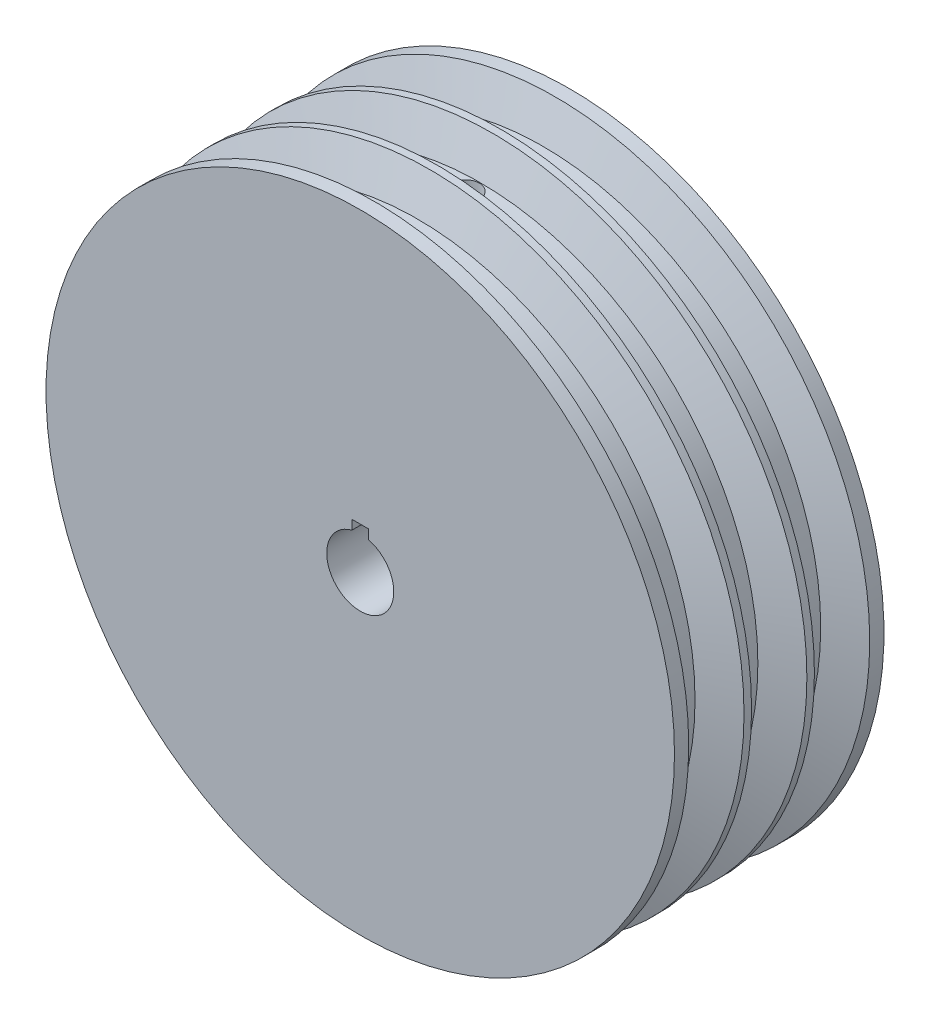
from build123d import *

# Parameters (mm, degrees)
SKETCH1_R           = 75
BOSS_EXTRUDE1_DEPTH = 40
SKETCH2_R           = 8
CUT_EXTRUDE1_DEPTH  = 150
SKETCH10_R          = 100
CUT_EXTRUDE5_DEPTH  = 20
SKETCH11_R          = 30
SKETCH11_R_2        = 8
BOSS_EXTRUDE2_DEPTH = 20
SKETCH12_R          = 130
CUT_EXTRUDE6_DEPTH  = 30
SKETCH13_W          = 4
SKETCH13_H          = 4
CUT_EXTRUDE7_DEPTH  = 500
SKETCH15_W          = 3.4
SKETCH15_H          = 65


with BuildPart() as part:
    # Sketch1 → Boss-Extrude1 (new, symmetric)
    with BuildSketch(Plane.XY):
        Circle(SKETCH1_R)
    extrude(amount=BOSS_EXTRUDE1_DEPTH, both=True)

    # Sketch2 → Cut-Extrude1 (cut)
    with BuildSketch(Plane.XY.offset(40)):
        Circle(SKETCH2_R)
    extrude(amount=-CUT_EXTRUDE1_DEPTH, mode=Mode.SUBTRACT)

    # Sketch4 → Cut-Revolve1 (revolve, cut)
    with BuildSketch(Plane(origin=(0, 0, 0), x_dir=(0, 0, -1), z_dir=(1, 0, 0)), mode=Mode.PRIVATE) as cut_revolve1_sk:
        Polygon((-40, 75), (-36.6, 75), (-33.604349764, 66.3), (-26.395650236, 66.3), (-23.4, 75), (-21.6, 75), (-18.604349764, 66.3), (-11.395650236, 66.3), (-8.4, 75), (-6.6, 75), (-3.604349764, 66.3), (3.604349764, 66.3), (6.6, 75), (10, 75), (10, 161.050459045), (-40, 161.050459045), align=None)
    revolve(cut_revolve1_sk.sketch.rotate(Axis((0, 0, 0), (0, 0, -1)), 90), axis=Axis((0, 0, 0), (0, 0, -1)), mode=Mode.SUBTRACT)

    # Sketch10 → Cut-Extrude5 (cut)
    with BuildSketch(Plane(origin=(0, 0, -40), x_dir=(-1, 0, 0), z_dir=(0, 0, -1))):
        Circle(SKETCH10_R)
    extrude(amount=-CUT_EXTRUDE5_DEPTH, mode=Mode.SUBTRACT)

    # Sketch11 → Boss-Extrude2 (add)
    with BuildSketch(Plane(origin=(0, 0, -20), x_dir=(-1, 0, 0), z_dir=(0, 0, -1))):
        Circle(SKETCH11_R)
        with Locations(Location((0, 0, 0), (0, 0, 180))):
            Circle(SKETCH11_R_2, mode=Mode.SUBTRACT)
    extrude(amount=BOSS_EXTRUDE2_DEPTH)

    # Sketch12 → Cut-Extrude6 (cut)
    with BuildSketch(Plane(origin=(0, 0, -40), x_dir=(-1, 0, 0), z_dir=(0, 0, -1))):
        Circle(SKETCH12_R)
    extrude(amount=-CUT_EXTRUDE6_DEPTH, mode=Mode.SUBTRACT)

    # Sketch13 → Cut-Extrude7 (cut)
    with BuildSketch(Plane(origin=(0, 0, -10), x_dir=(-1, 0, 0), z_dir=(0, 0, -1))):
        with Locations((0, 8)):
            Rectangle(SKETCH13_W, SKETCH13_H)
    extrude(amount=-CUT_EXTRUDE7_DEPTH, mode=Mode.SUBTRACT)

    # Sketch15 → M8 Tapped Hole1 (revolve, cut)
    with BuildSketch(Plane(origin=(0, 10, 15), x_dir=(0, 0, -1), z_dir=(1, 0, 0))):
        with Locations((1.7, 32.5)):
            Rectangle(SKETCH15_W, SKETCH15_H)
    revolve(axis=Axis((0, 3.65, 15), (0, 1, 0)), mode=Mode.SUBTRACT)


solid = part.part
